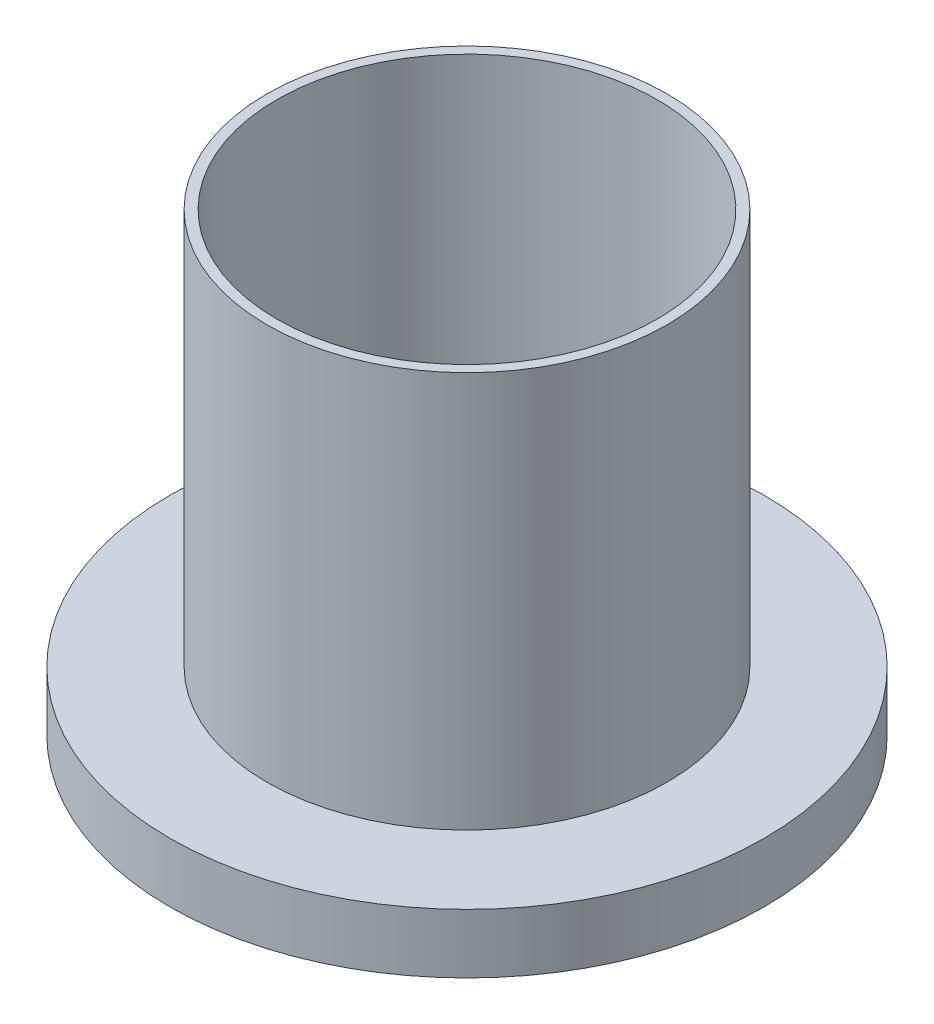
SolidWorks part; units mm, degrees
ref_plane "Front Plane" through (0, 0, 0) normal (0, 0, 1) x (1, 0, 0)
ref_plane "Top Plane" through (0, 0, 0) normal (0, 1, 0) x (1, 0, 0)
ref_plane "Right Plane" through (0, 0, 0) normal (1, 0, 0) x (0, 0, -1)
sketch "Sketch1" plane through (0, 0, 0) normal (0, 1, 0) x (1, 0, 0)
  circle A0 centre (0, 0) radius 10.1
  dimension "D1" = 20.2
extrude "Boss-Extrude1" add sketch "Sketch1" along normal blind 20
sketch "Sketch2" plane through (0, 0, 0) normal (0, -1, 0) x (1, 0, 0)
  circle A0 centre (0, 0) radius 15
extrude "Boss-Extrude2" add sketch "Sketch2" against normal blind 3 from offset 3
sketch "Sketch4" plane through (0, 20, 0) normal (0, 1, 0) x (1, 0, 0)
  circle A0 centre (0, 0) radius 9.6
extrude "Cut-Extrude1" cut sketch "Sketch4" against normal through all
